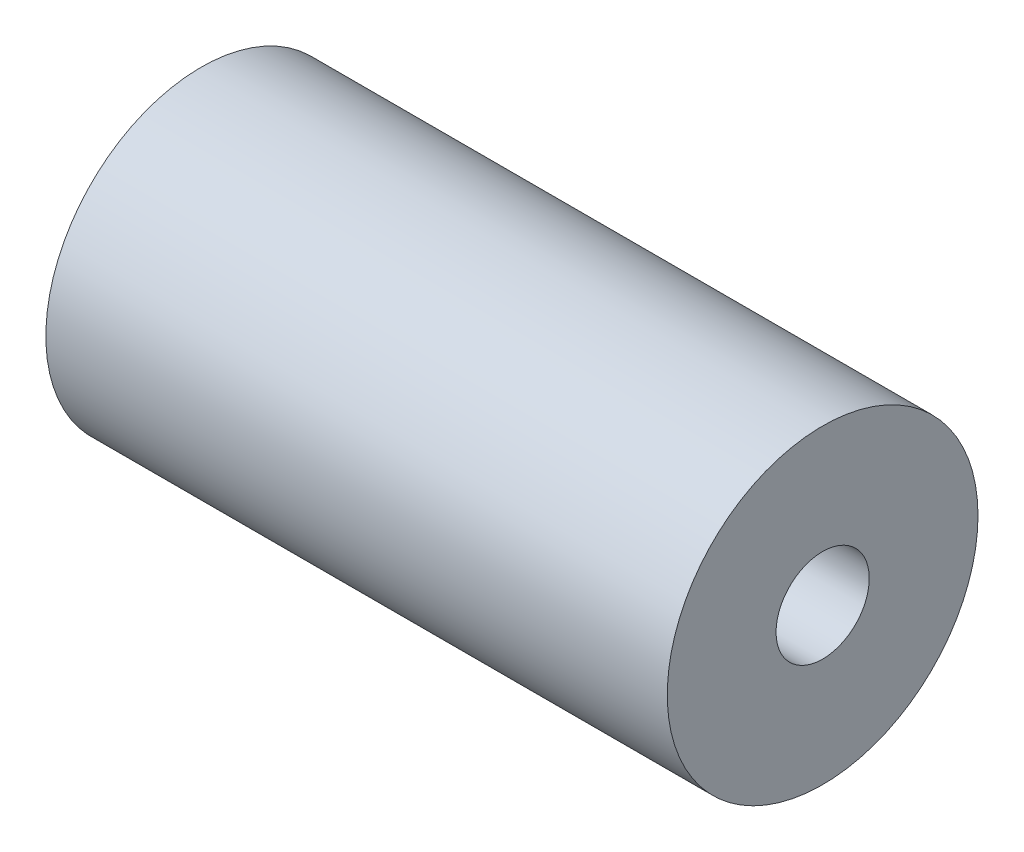
SolidWorks part; units mm, degrees
ref_plane "前视基准面" through (0, 0, 0) normal (0, 0, 1) x (1, 0, 0)
ref_plane "上视基准面" through (0, 0, 0) normal (0, 1, 0) x (1, 0, 0)
ref_plane "右视基准面" through (0, 0, 0) normal (1, 0, 0) x (0, 0, -1)
sketch "草图1" plane through (0, 0, 0) normal (1, 0, 0) x (0, 0, -1)
  circle A0 centre (0, 0) radius 10
  circle A1 centre (0, 0) radius 3
extrude "凸台-拉伸1" add sketch "草图1" along normal blind 40
sketch "草图3" plane through (0, 0, 0) normal (-1, 0, 0) x (0, 0, 1)
  circle A0 centre (0, 0) radius 7.5
  circle A1 centre (0, 0) radius 3
extrude "凸台-拉伸2" add sketch "草图3" along normal blind 1
